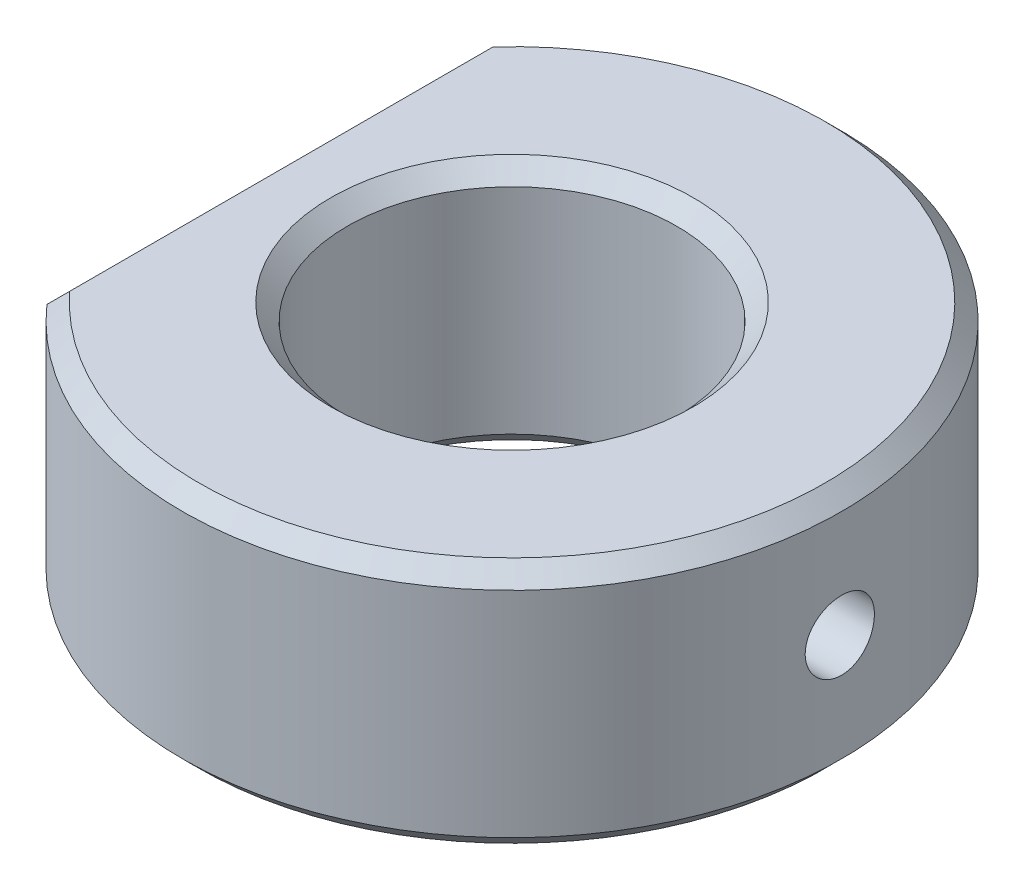
from build123d import *

# Parameters (mm, degrees)
SKETCH_1_R          = 20
SKETCH_1_R_2        = 10
EXTRUDE_1_DEPTH     = 15
SKETCH_2_W          = 9.046336772
SKETCH_2_H          = 38.953764593
CUT_EXTRUDE_1_DEPTH = 33.015621187
CHAMFER_1_SIZE      = 1
SKETCH_3_W          = 2.1
SKETCH_3_H          = 20


with BuildPart() as part:
    # 草图1 → 凸台-拉伸1 (new body)
    with BuildSketch(Plane(origin=(0, 0, 0), x_dir=(1, 0, 0), z_dir=(0, 1, 0))):
        with Locations(Location((0, 0, 0), (0, 0, 270))):
            Circle(SKETCH_1_R)
        with Locations(Location((0, 0, 0), (0, 0, 270))):
            Circle(SKETCH_1_R_2, mode=Mode.SUBTRACT)
    extrude(amount=EXTRUDE_1_DEPTH)

    # 草图2 → 切除-拉伸1 (cut, through all)
    with BuildSketch(Plane(origin=(0, 15, 0), x_dir=(1, 0, 0), z_dir=(0, 1, 0))):
        with Locations((-19.523168386, 4.341186033)):
            Rectangle(SKETCH_2_W, SKETCH_2_H)
    extrude(amount=-CUT_EXTRUDE_1_DEPTH, mode=Mode.SUBTRACT)

    # 倒角1
    chamfer_1_edges = [part.edges().sort_by_distance(p)[0] for p in [
        (20, 15, 0),
        (20, 0, 0),
        (-15, 0, 0),
        (-15, 15, 0),
        (0, 0, -10),
        (0, 15, -10),
    ]]
    chamfer(chamfer_1_edges, length=CHAMFER_1_SIZE)

    # 草图3 → M5 螺纹孔1 (revolve, cut)
    with BuildSketch(Plane.ZX.offset(7.5)):
        with Locations((1.05, 10)):
            Rectangle(SKETCH_3_W, SKETCH_3_H)
    revolve(axis=Axis((-6.35, 7.5, 0), (1, 0, 0)), mode=Mode.SUBTRACT)


solid = part.part
